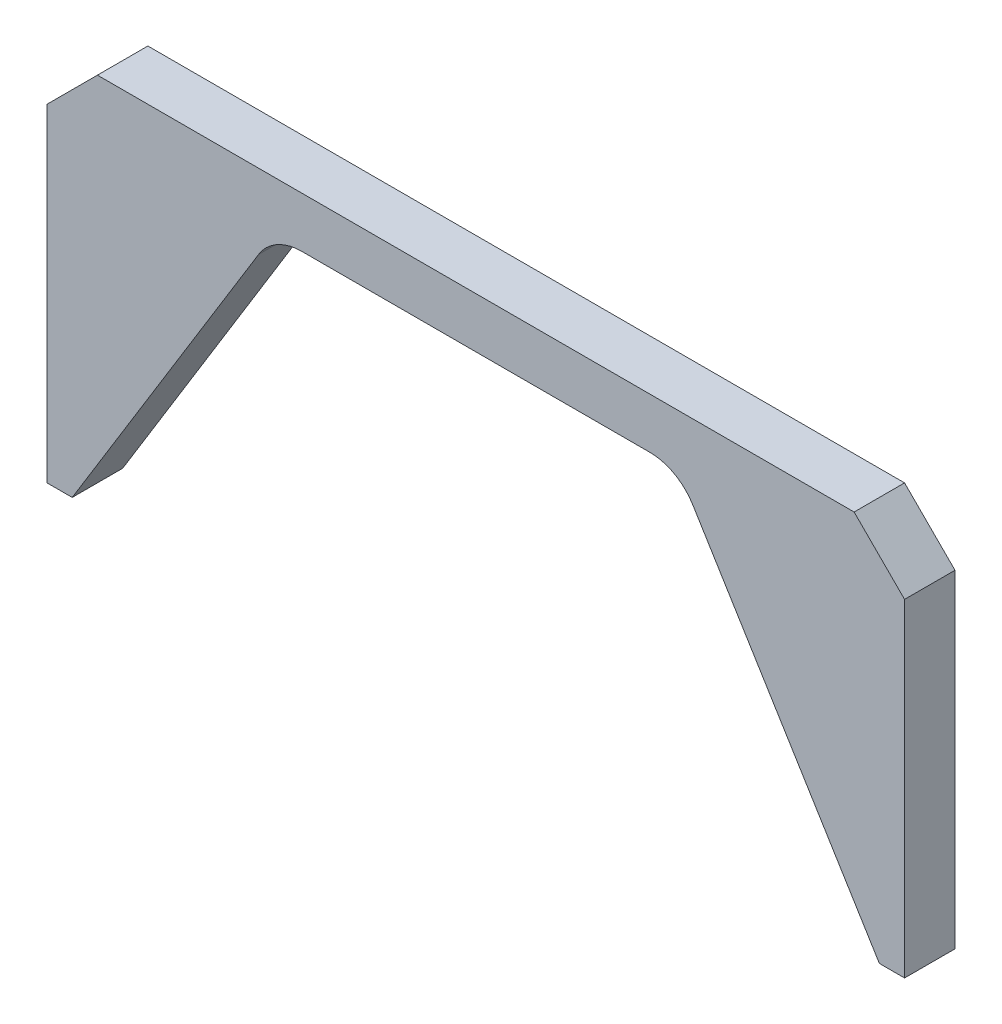
from build123d import *

# Parameters (mm, degrees)
BOSS_EXTRUDE1_DEPTH = 5
CHAMFER1_SIZE       = 10


with BuildPart() as part:
    # Sketch1 → Boss-Extrude1 (new, symmetric)
    with BuildSketch(Plane.XY):
        with BuildLine():
            Line((-85, 0), (-80, 0))
            Line((-80, 0), (-43.022132459, 60.231945943))
            ThreePointArc((-43.022132459, 60.231945943), (-39.382649924, 63.726954206), (-34.5, 65))
            Line((-34.5, 65), (34.5, 65))
            ThreePointArc((34.5, 65), (39.382649924, 63.726954206), (43.022132459, 60.231945943))
            Line((43.022132459, 60.231945943), (80, 0))
            Line((80, 0), (85, 0))
            Line((85, 0), (85, 75))
            Line((85, 75), (-85, 75))
            Line((-85, 75), (-85, 0))
        make_face()
    extrude(amount=BOSS_EXTRUDE1_DEPTH, both=True)

    # Chamfer1
    chamfer1_edges = [part.edges().sort_by_distance(p)[0] for p in [
        (-85, 75, 0),
        (85, 75, 0),
    ]]
    chamfer(chamfer1_edges, length=CHAMFER1_SIZE)


solid = part.part
